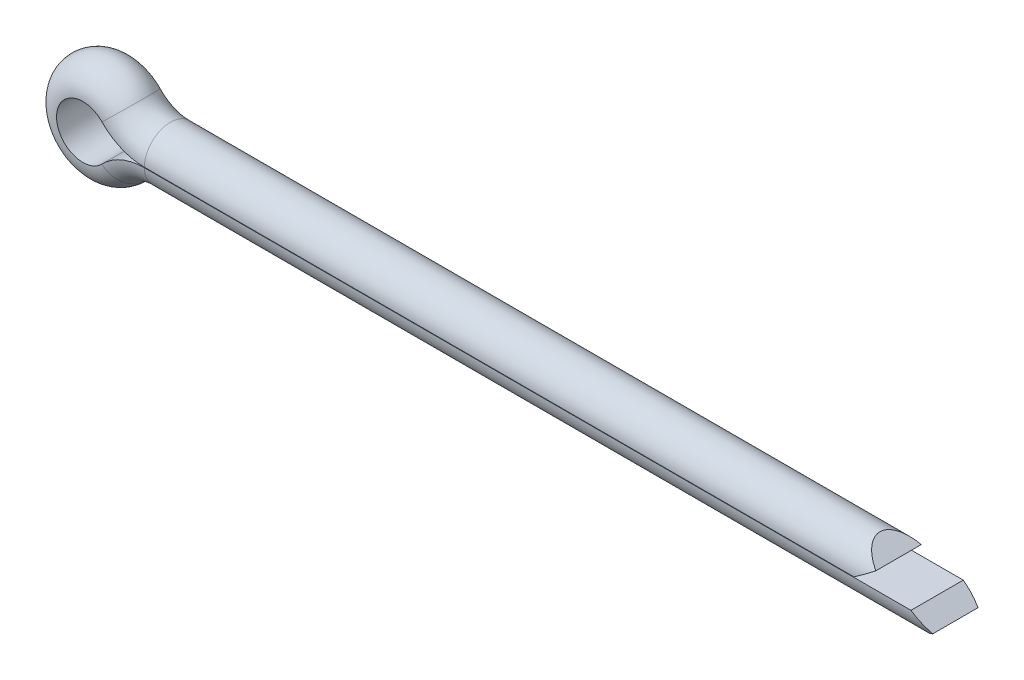
from build123d import *

# Parameters (mm, degrees)
CUT_EXTRUDE1_DEPTH      = 38.288770437
CUT_EXTRUDE1_DEPTH_BACK = 38.288770437


with BuildPart() as part:
    # Sweep2: sweep along a path in Dimension sketch
    with BuildLine(Plane.XY) as sweep2_path:
        Line((34.7, 1.15), (2.7, 1.15))
        ThreePointArc((2.7, 1.15), (2.133929691, 1.265530578), (1.658403483, 1.593642961))
        ThreePointArc((1.658403483, 1.593642961), (-2.3, 0), (1.658403483, -1.593642961))
        ThreePointArc((1.658403483, -1.593642961), (2.133929691, -1.265530578), (2.7, -1.15))
        Line((2.7, -1.15), (37.2, -1.15))
    # Sketch2 → Sweep2 (sweep)
    with BuildSketch(Plane(origin=(34.7, 1.15, 0), x_dir=(0, 0, 1), z_dir=(-1, 0, 0))):
        with BuildLine():
            Line((-1.149956521, -1.14), (1.149956521, -1.14))
            ThreePointArc((1.149956521, -1.14), (0, 0), (-1.149956521, -1.14))
        make_face()
    sweep(path=sweep2_path.line)

    # Sketch3 → Cut-Extrude1 (cut, two sides: drawn at the far end of the back side and taken through both)
    with BuildSketch(Plane.XY.offset(-CUT_EXTRUDE1_DEPTH_BACK)):
        Polygon((34.7, 0.57), (33.882315934, 1.15), (37.21, 1.15), (37.21, -1.15), (36.375313858, -1.15), (37.2, -0.58), (36.382315934, 0), (33.875313858, 0), align=None)
    extrude(amount=CUT_EXTRUDE1_DEPTH + CUT_EXTRUDE1_DEPTH_BACK, mode=Mode.SUBTRACT)


solid = part.part
